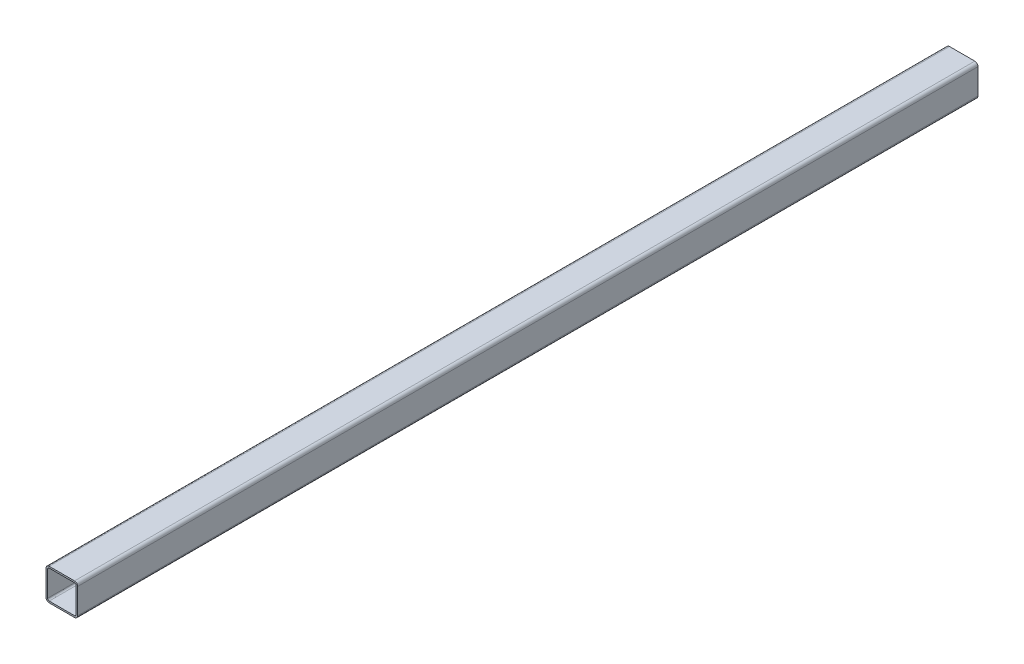
SolidWorks part; units mm, degrees
material "普通碳钢"
ref_plane "Front Plane" through (0, 0, 0) normal (0, 0, 1) x (1, 0, 0)
ref_plane "Top Plane" through (0, 0, 0) normal (0, 1, 0) x (1, 0, 0)
ref_plane "Right Plane" through (0, 0, 0) normal (1, 0, 0) x (0, 0, -1)
sketch "Sketch1" plane through (0, 0, 0) normal (0, 0, 1) x (1, 0, 0)
  line L0 (10, 95) -> (90, 95)
  line L1 (10, 0) -> (90, 0)
  line L2 (0, 10) -> (0, 90)
  line L3 (10, 100) -> (90, 100)
  line L4 (100, 10) -> (100, 90)
  line L5 (95, 10) -> (95, 90)
  line L6 (10, 5) -> (90, 5)
  line L7 (5, 10) -> (5, 90)
  arc A0 (100, 10) -> (90, 0) centre (90, 10) cw
  arc A1 (0, 90) -> (10, 100) centre (10, 90) cw
  arc A2 (100, 90) -> (90, 100) centre (90, 90) ccw
  arc A3 (10, 0) -> (0, 10) centre (10, 10) cw
  arc A4 (95, 90) -> (90, 95) centre (90, 90) ccw
  arc A5 (95, 10) -> (90, 5) centre (90, 10) cw
  arc A6 (10, 5) -> (5, 10) centre (10, 10) cw
  arc A7 (5, 90) -> (10, 95) centre (10, 90) cw
  point P7 (100, 0)
  point P10 (0, 100)
  point P13 (100, 100)
  point P16 (0, 0)
  dimension "D3" = 10
  dimension "D4" = 10
  dimension "D5" = 10
  dimension "D6" = 10
  dimension "D1" = 100
  dimension "D2" = 100
  dimension "D7" = 5
extrude "Boss-Extrude1" add sketch "Sketch1" along normal blind 2840
